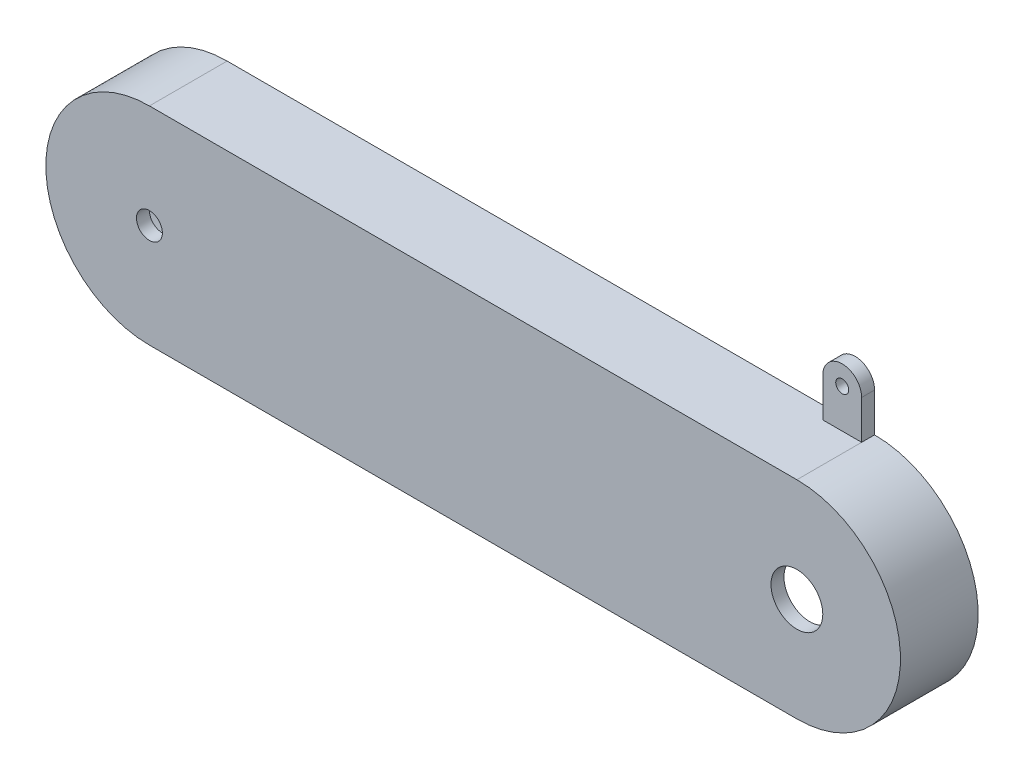
SolidWorks part; units mm, degrees
ref_plane "前视基准面" through (0, 0, 0) normal (0, 0, 1) x (1, 0, 0)
ref_plane "上视基准面" through (0, 0, 0) normal (0, 1, 0) x (1, 0, 0)
ref_plane "右视基准面" through (0, 0, 0) normal (1, 0, 0) x (0, 0, -1)
sketch "草图1" plane through (0, 0, 0) normal (0, 0, 1) x (1, 0, 0)
  line L0 (0, 80) -> (-500, 80)
  line L2 (-500, -80) -> (0, -80)
  arc A0 (0, -80) -> (0, 80) centre (0, 0) ccw
  circle A2 centre (0, 0) radius 20
  arc A7 (-500, 80) -> (-500, -80) centre (-500, 0) ccw
  circle A8 centre (-500, 0) radius 10
extrude "凸台-拉伸1" add sketch "草图1" along normal blind 10
sketch "草图2" plane through (0, 0, 0) normal (0, 0, -1) x (-1, 0, 0)
  line L0 (0, -70) -> (500, -70)
  line L1 (500, 70) -> (0, 70)
  line L2 (0, -80) -> (500, -80)
  line L3 (500, 80) -> (0, 80)
  line L4 (0, -80) -> (500, -80)
  line L5 (500, 80) -> (0, 80)
  arc A0 (500, -70) -> (500, 70) centre (500, 0) ccw
  arc A1 (0, 70) -> (0, -70) centre (0, 0) ccw
  arc A2 (0, 80) -> (0, -80) centre (0, 0) ccw
  arc A3 (500, -80) -> (500, 80) centre (500, 0) ccw
  arc A4 (0, 80) -> (0, -80) centre (0, 0) ccw
  arc A5 (500, -80) -> (500, 80) centre (500, 0) ccw
  dimension "D1" = 0
  dimension "D2" = 10
extrude "凸台-拉伸2" add sketch "草图2" along normal blind 50
sketch "草图4" plane through (0, 0, -50) normal (0, 0, -1) x (-1, 0, 0)
  line L0 (500, 80) -> (0, 80) construction
  line L2 (0, 110) -> (0, 80)
  line L3 (0, 80) -> (30, 80)
  line L4 (30, 110) -> (30, 80)
  arc A0 (30, 110) -> (0, 110) centre (15, 110) ccw
  circle A1 centre (15, 110) radius 5
  dimension "D4" = 15
  dimension "D2" = 10
  dimension "D1" = 30
  dimension "D3" = 30
extrude "凸台-拉伸3" add sketch "草图4" against normal blind 10
